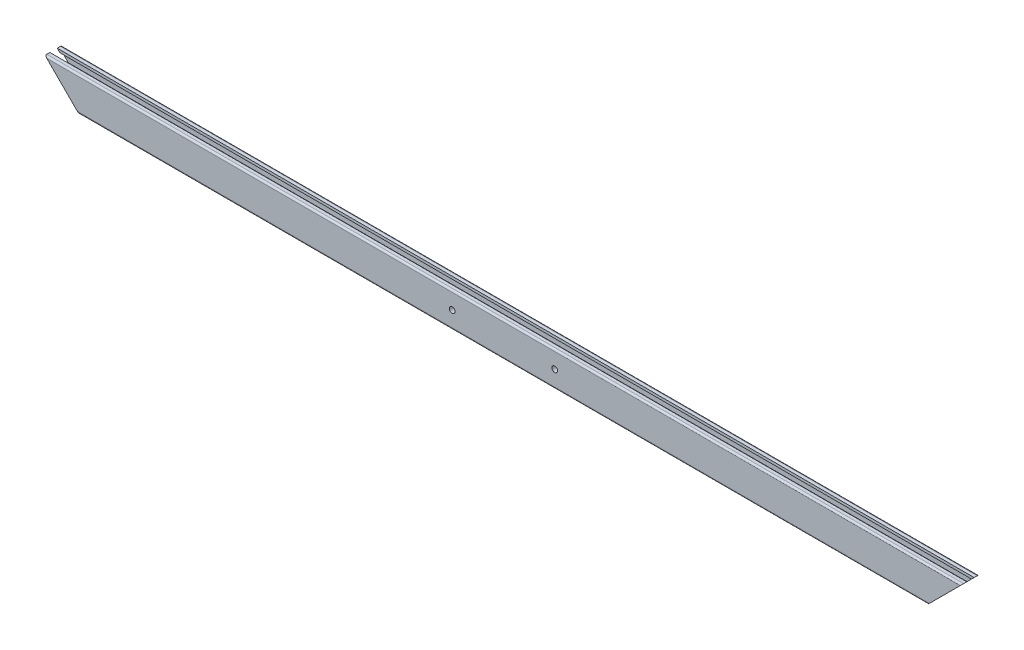
SolidWorks part; units mm, degrees
ref_plane "前视" through (0, 0, 0) normal (0, 0, 1) x (1, 0, 0)
ref_plane "上视" through (0, 0, 0) normal (0, 1, 0) x (1, 0, 0)
ref_plane "右视" through (0, 0, 0) normal (1, 0, 0) x (0, 0, -1)
sketch3d "3D草图1"
  line L0 (-402.5, 0, 0) -> (402.5, 0, 0)
  dimension "D1" = 805
other "结构构件1"
ref_plane "基准面1" through (-402.5, 0, 0) normal (1, 0, 0) x (0, 0, -1)
sketch "Sketch11" plane through (-402.5, 0, 0) normal (1, 0, 0) x (0, 0, -1)
  line L1 (0, 16.311) -> (0, -16.311) construction
  line L2 (0, 0) -> (9.513, 0) construction
  line L3 (-6, -15) -> (-3.25, -15)
  line L4 (-7.5, -13.5) -> (-7.5, 13.5)
  line L5 (-6, 15) -> (-3.25, 15)
  line L6 (7.5, -13.5) -> (7.5, 13.5)
  line L17 (3.25, 15) -> (6, 15)
  line L20 (-5, 12.7) -> (-5, 7)
  line L21 (-3.25, 12.7) -> (-5, 12.7)
  line L24 (5, 12.7) -> (5, 7)
  line L25 (3.25, 12.7) -> (5, 12.7)
  line L26 (-3.25, 15) -> (-3.25, 12.7)
  line L27 (3.25, 15) -> (3.25, 12.7)
  line L40 (5, -12.7) -> (5, -7)
  line L41 (3.25, -12.7) -> (5, -12.7)
  line L44 (-5, -12.7) -> (-5, -7)
  line L45 (-3.25, -12.7) -> (-5, -12.7)
  line L47 (3.25, -15) -> (3.25, -12.7)
  line L48 (-3.25, -15) -> (-3.25, -12.7)
  line L49 (3.25, -15) -> (6, -15)
  arc A0 (-6, -15) -> (-7.5, -13.5) centre (-6, -13.5) cw
  arc A1 (6, -15) -> (7.5, -13.5) centre (6, -13.5) ccw
  arc A2 (6, 15) -> (7.5, 13.5) centre (6, 13.5) cw
  arc A3 (-7.5, 13.5) -> (-6, 15) centre (-6, 13.5) cw
  circle A4 centre (0, 0) radius 2.5
  arc A5 (-5, 7) -> (5, 7) centre (0, 10.3166) ccw
  arc A6 (-5, -7) -> (5, -7) centre (0, -10.3166) cw
  point P4 (0, 0)
  point P21 (0, 0)
  point P44 (-7.5, 15)
  point P45 (7.5, 15)
  point P46 (7.5, -15)
  point P47 (-7.5, -15)
  point P48 (0, -15)
  point P49 (0, 15)
  dimension "D1" = 30
  dimension "D2" = 15
  dimension "D3" = 1.5
  dimension "D4" = 5
  dimension "D5" = 6.5
  dimension "D6" = 6
  dimension "D7" = 8
  dimension "D8" = 10
  dimension "D9" = 2.3
sketch "草图4" plane through (0, 0, 7.5) normal (0, 0, 1) x (1, 0, 0)
  line L0 (-402.5, 15) -> (-372.5, -15)
  line L1 (402.5, -15) -> (-402.5, -15) construction
  line L2 (0, 0) -> (0, -85.0329) construction
  line L3 (-372.5, -15) -> (-402.5, -15)
  line L4 (-402.5, -15) -> (-402.5, 15)
  line L5 (402.5, -15) -> (402.5, 15)
  line L6 (372.5, -15) -> (402.5, -15)
  line L7 (402.5, 15) -> (372.5, -15)
extrude "切除-拉伸1" cut sketch "草图4" against normal through all
hole_wizard "M6 螺纹孔1" positions "草图7" profile "草图6" tap size "M6" standard "Iso" end condition through all
sketch "草图7" plane through (0, 0, 7.5) normal (0, 0, 1) x (1, 0, 0)
  line L0 (0, 0) -> (0, -34.9561) construction
  point P0 (-45, 0)
  point P8 (45, 0)
  dimension "D1" = 90
cosmetic thread "孔螺蚊线1" parameters "D2"=6
cosmetic thread "孔螺蚊线2" parameters "D2"=6
sketch "草图6" plane through (-45, 0, 7.5) normal (1, 0, 0) x (0, -1, 0)
  line L0 (0, 0) -> (0, 15)
  line L1 (0, 15) -> (2.5, 15)
  line L2 (2.5, 15) -> (2.5, 0)
  line L5 (2.5, 0) -> (0, 0)
  line L11 (0, -6.35) -> (0, 107.95) construction
  dimension "通孔螺纹孔钻头直径" = 5
  dimension "通孔螺纹孔钻头深度" = 15
